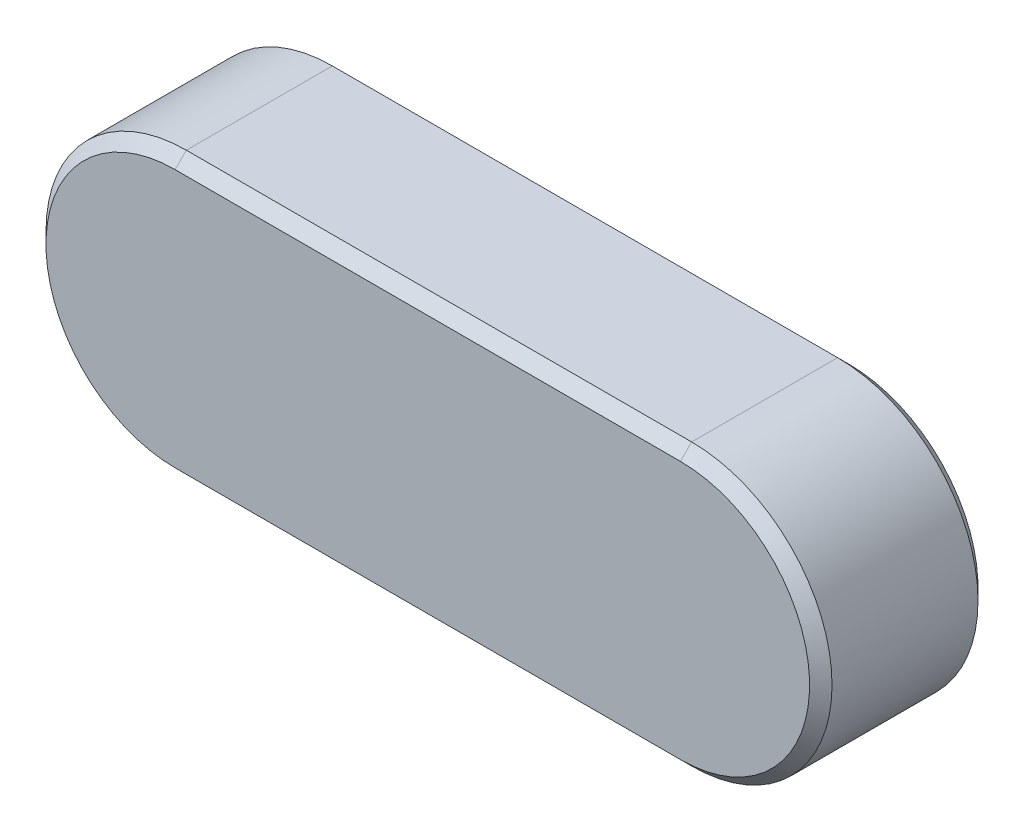
SolidWorks part; units mm, degrees
ref_plane "Front" through (0, 0, 0) normal (0, 0, 1) x (1, 0, 0)
ref_plane "Top" through (0, 0, 0) normal (0, 1, 0) x (1, 0, 0)
ref_plane "Right" through (0, 0, 0) normal (1, 0, 0) x (0, 0, -1)
sketch "Sketch1" plane through (0, 0, 0) normal (0, 0, 1) x (1, 0, 0)
  line L0 (-36, 10) -> (0, 10)
  line L1 (0, -10) -> (-36, -10)
  arc A0 (0, 10) -> (0, -10) centre (0, 0) cw
  arc A1 (-36, -10) -> (-36, 10) centre (-36, 0) cw
  dimension "L" = 56
  dimension "b" = 20
extrude "BaseKey" add sketch "Sketch1" along normal mid plane 12
sketch "Sketch2" plane through (0, 0, 0) normal (0, 0, 1) x (1, 0, 0)
  line L1 (-46, 10) -> (10, 10)
  line L2 (-46, 10) -> (-46, -10)
  line L3 (-46, -10) -> (10, -10)
  line L4 (10, 10) -> (10, -10)
  line L6 (0, -10) -> (-36, -10) construction
  line L7 (-36, 10) -> (0, 10) construction
  arc A2 (0, -10) -> (0, 10) centre (0, 0) ccw construction
  arc A3 (-36, 10) -> (-36, -10) centre (-36, 0) ccw construction
extrude "Extrude1" [suppressed] add sketch "Sketch2" along normal mid plane 12
sketch "Sketch3" plane through (0, 0, 0) normal (0, 0, 1) x (1, 0, 0)
  line L0 (10, 10) -> (-36, 10)
  line L1 (-36, -10) -> (10, -10)
  line L2 (10, -10) -> (10, 10)
  line L5 (-36, 10) -> (0, 10) construction
  arc A0 (-36, 10) -> (-36, -10) centre (-36, 0) ccw
  arc A1 (0, -10) -> (0, 10) centre (0, 0) ccw construction
  arc A4 (-36, 10) -> (-36, -10) centre (-36, 0) ccw construction
extrude "Extrude2" [suppressed] add sketch "Sketch3" along normal mid plane 12
chamfer "Chamfer1" distance 0.8 angle 45 8 edges at (10, 0, -6) (-18, -10, -6) (-46, 0, -6) (-18, 10, -6) (-46, 0, 6) (-18, -10, 6) (10, 0, 6) (-18, 10, 6)
equation "\"D1@Extrude1\"=\"h@BaseKey\""
equation "\"D1@Extrude2\"=\"h@BaseKey\""
